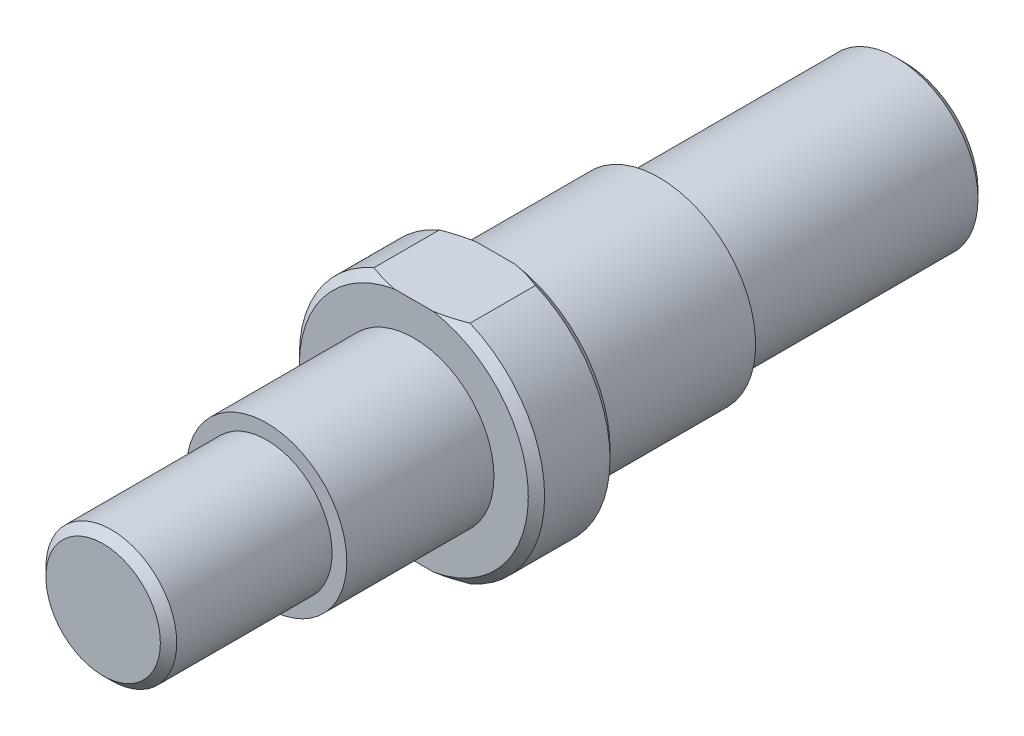
from build123d import *

# Parameters (mm, degrees)
SKETCH_1_R          = 7.5
EXTRUDE_1_DEPTH     = 24.5
SKETCH_2_OUTSIDE_W  = 27.678
SKETCH_2_OUTSIDE_H  = 27.678
SKETCH_2_OUTSIDE_R  = 4.9
CUT_EXTRUDE_1_DEPTH = 19
SKETCH_3_OUTSIDE_W  = 27.678
SKETCH_3_OUTSIDE_H  = 27.678
SKETCH_3_OUTSIDE_R  = 4
CUT_EXTRUDE_2_DEPTH = 10
SKETCH_4_OUTSIDE_W  = 27.678
SKETCH_4_OUTSIDE_H  = 27.678
SKETCH_4_OUTSIDE_R  = 5.9
CUT_EXTRUDE_3_DEPTH = 25
SKETCH_5_OUTSIDE_W  = 27.678
SKETCH_5_OUTSIDE_H  = 27.678
SKETCH_5_OUTSIDE_R  = 5
CUT_EXTRUDE_4_DEPTH = 15
CHAMFER_1_SIZE      = 0.5
SKETCH_6_W          = 15
SKETCH_6_H          = 6
CUT_EXTRUDE_5_DEPTH = 15


with BuildPart() as part:
    # 草图1 → 凸台-拉伸1 (new, symmetric)
    with BuildSketch(Plane.XY):
        Circle(SKETCH_1_R)
    extrude(amount=EXTRUDE_1_DEPTH, both=True)

    # 草图2 outside → 切除-拉伸1 (cut)
    with BuildSketch(Plane.XY.offset(24.5)):
        Rectangle(SKETCH_2_OUTSIDE_W, SKETCH_2_OUTSIDE_H)
        Circle(SKETCH_2_OUTSIDE_R, mode=Mode.SUBTRACT)
    extrude(amount=-CUT_EXTRUDE_1_DEPTH, mode=Mode.SUBTRACT)

    # 草图3 outside → 切除-拉伸2 (cut)
    with BuildSketch(Plane.XY.offset(24.5)):
        Rectangle(SKETCH_3_OUTSIDE_W, SKETCH_3_OUTSIDE_H)
        Circle(SKETCH_3_OUTSIDE_R, mode=Mode.SUBTRACT)
    extrude(amount=-CUT_EXTRUDE_2_DEPTH, mode=Mode.SUBTRACT)

    # 草图4 outside → 切除-拉伸3 (cut)
    with BuildSketch(Plane(origin=(0, 0, -24.5), x_dir=(-1, 0, 0), z_dir=(0, 0, -1))):
        Rectangle(SKETCH_4_OUTSIDE_W, SKETCH_4_OUTSIDE_H)
        Circle(SKETCH_4_OUTSIDE_R, mode=Mode.SUBTRACT)
    extrude(amount=-CUT_EXTRUDE_3_DEPTH, mode=Mode.SUBTRACT)

    # 草图5 outside → 切除-拉伸4 (cut)
    with BuildSketch(Plane(origin=(0, 0, -24.5), x_dir=(-1, 0, 0), z_dir=(0, 0, -1))):
        Rectangle(SKETCH_5_OUTSIDE_W, SKETCH_5_OUTSIDE_H)
        Circle(SKETCH_5_OUTSIDE_R, mode=Mode.SUBTRACT)
    extrude(amount=-CUT_EXTRUDE_4_DEPTH, mode=Mode.SUBTRACT)

    # 倒角1
    chamfer_1_edges = [part.edges().sort_by_distance(p)[0] for p in [
        (-4, 0, 24.5),
        (-7.5, 0, 0.5),
        (5, 0, -24.5),
        (-7.5, 0, 5.5),
    ]]
    chamfer(chamfer_1_edges, length=CHAMFER_1_SIZE)

    # 草图6 → 切除-拉伸5 (cut)
    with BuildSketch(Plane.XY.offset(5.5)):
        with Locations((0, 9.9)):
            Rectangle(SKETCH_6_W, SKETCH_6_H)
        with Locations((0, -9.9)):
            Rectangle(SKETCH_6_W, SKETCH_6_H)
    extrude(amount=-CUT_EXTRUDE_5_DEPTH, mode=Mode.SUBTRACT)


solid = part.part
